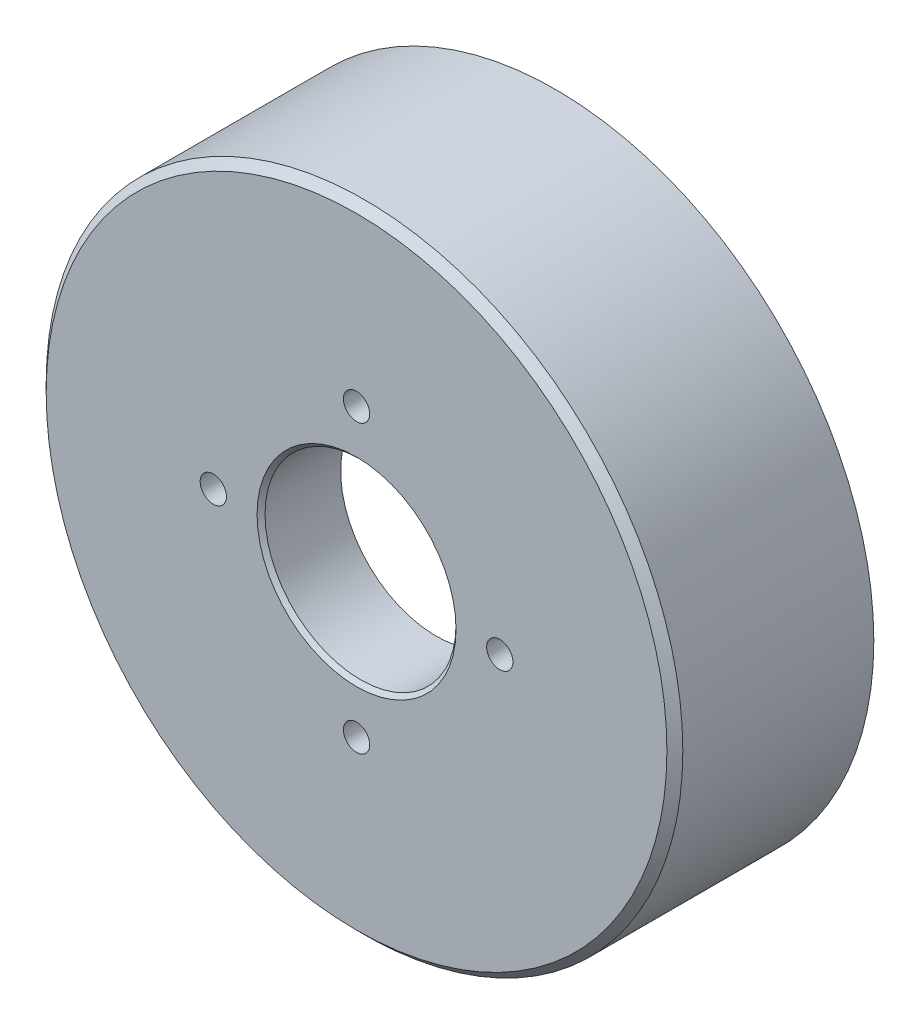
SolidWorks part; units mm, degrees
material "POM acetal copolymer"
ref_plane "Front Plane" through (0, 0, 0) normal (0, 0, 1) x (1, 0, 0)
ref_plane "Top Plane" through (0, 0, 0) normal (0, 1, 0) x (1, 0, 0)
ref_plane "Right Plane" through (0, 0, 0) normal (1, 0, 0) x (0, 0, -1)
sketch "Sketch8" plane through (0, 0, 0) normal (1, 0, 0) x (0, 0, -1)
  line L0 (0, 0) -> (109.5855, 0) construction
  line L1 (0, 0) -> (0, 40)
  line L2 (0, 40) -> (25, 40)
  line L3 (25, 40) -> (25, 35)
  line L4 (25, 35) -> (10, 35)
  line L5 (10, 35) -> (10, 0)
  line L6 (0, 0) -> (10, 0)
  dimension "D1" = 80
  dimension "D2" = 70
  dimension "D3" = 10
  dimension "D4" = 25
revolve "Revolve2" add sketch "Sketch8" angle 360 about L0
chamfer "Chamfer1" distance 1 angle 45 1 edges at (40, 0, 0)
sketch "Sketch9" plane through (0, 0, 0) normal (0, 0, 1) x (1, 0, 0)
  circle A0 centre (0, 0) radius 12
  dimension "D1" = 24
extrude "Cut-Extrude1" cut sketch "Sketch9" against normal through all
sketch "Sketch10" plane through (0, 0, 0) normal (0, 0, 1) x (1, 0, 0)
  line L0 (0, 18) -> (0, -18) construction
  line L1 (-18, 0) -> (18, 0) construction
  circle A0 centre (0, 0) radius 18
  dimension "D1" = 36
hole_wizard "M4 Tapped Hole1" positions "3DSketch1" profile "Sketch11" tap size "M4" standard "GB" end condition through all
sketch3d "3DSketch1"
  point P0 (0, 18, 0)
  point P3 (-18, 0, 0)
  point P6 (18, 0, 0)
  point P9 (0, -18, 0)
sketch "Sketch11" plane through (0, 18, 0) normal (1, 0, 0) x (0, -1, 0)
  line L0 (0, 0) -> (0, 25)
  line L1 (0, 25) -> (1.65, 25)
  line L2 (1.65, 25) -> (1.65, 0)
  line L5 (1.65, 0) -> (0, 0)
  line L11 (0, -6.35) -> (0, 107.95) construction
  dimension "通孔螺纹孔钻头直径" = 3.3
  dimension "通孔螺纹孔钻头深度" = 25
cosmetic thread "Cosmetic Thread1" parameters "D1"=8, "D2"=4.3
cosmetic thread "Cosmetic Thread2" parameters "D1"=8, "D2"=4.3
cosmetic thread "Cosmetic Thread3" parameters "D1"=8, "D2"=4.3
cosmetic thread "Cosmetic Thread4" parameters "D1"=8, "D2"=4.3
chamfer "Chamfer2" distance 0.5 angle 45 1 edges at (12, 0, 0)
